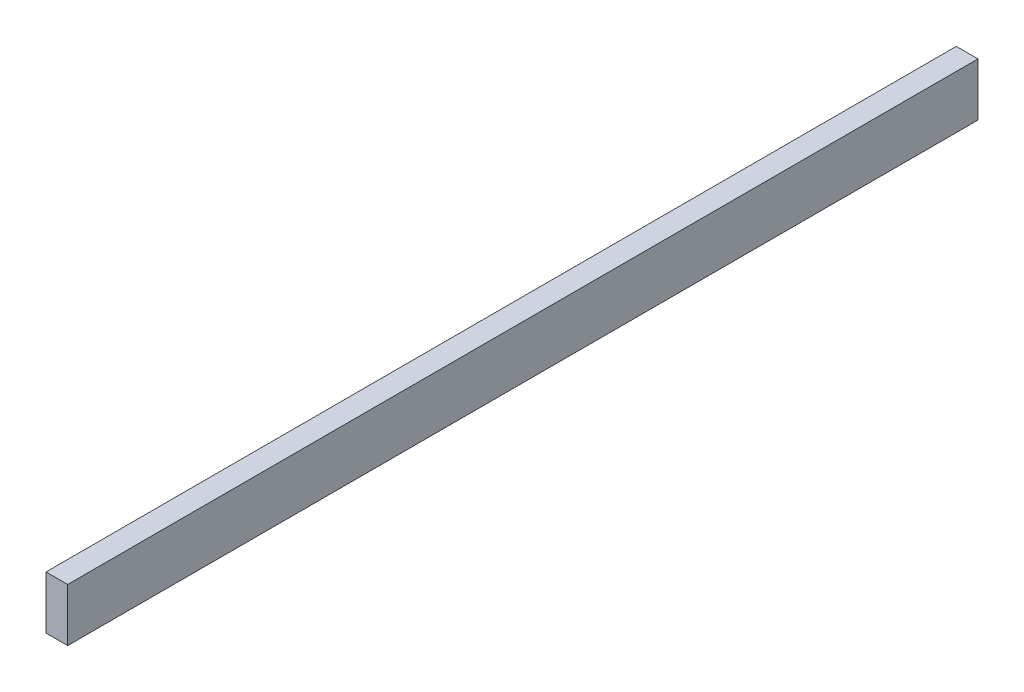
SolidWorks part; units mm, degrees
material "Q235-A"
ref_plane "Front Plane" through (0, 0, 0) normal (0, 0, 1) x (1, 0, 0)
ref_plane "Top Plane" through (0, 0, 0) normal (0, 1, 0) x (1, 0, 0)
ref_plane "Right Plane" through (0, 0, 0) normal (1, 0, 0) x (0, 0, -1)
sketch "Sketch1" plane through (0, 0, 0) normal (1, 0, 0) x (0, 0, -1)
  line L1 (945, -55) -> (-945, -55)
  line L2 (945, -55) -> (945, 55)
  line L3 (945, 55) -> (-945, 55)
  line L4 (-945, -55) -> (-945, 55)
  line L5 (945, -55) -> (-945, 55) construction
  line L6 (945, 55) -> (-945, -55) construction
  point P0 (0, 0)
  dimension "D1" = 1890
  dimension "D2" = 110
extrude "Boss-Extrude1" add sketch "Sketch1" along normal mid plane 45
